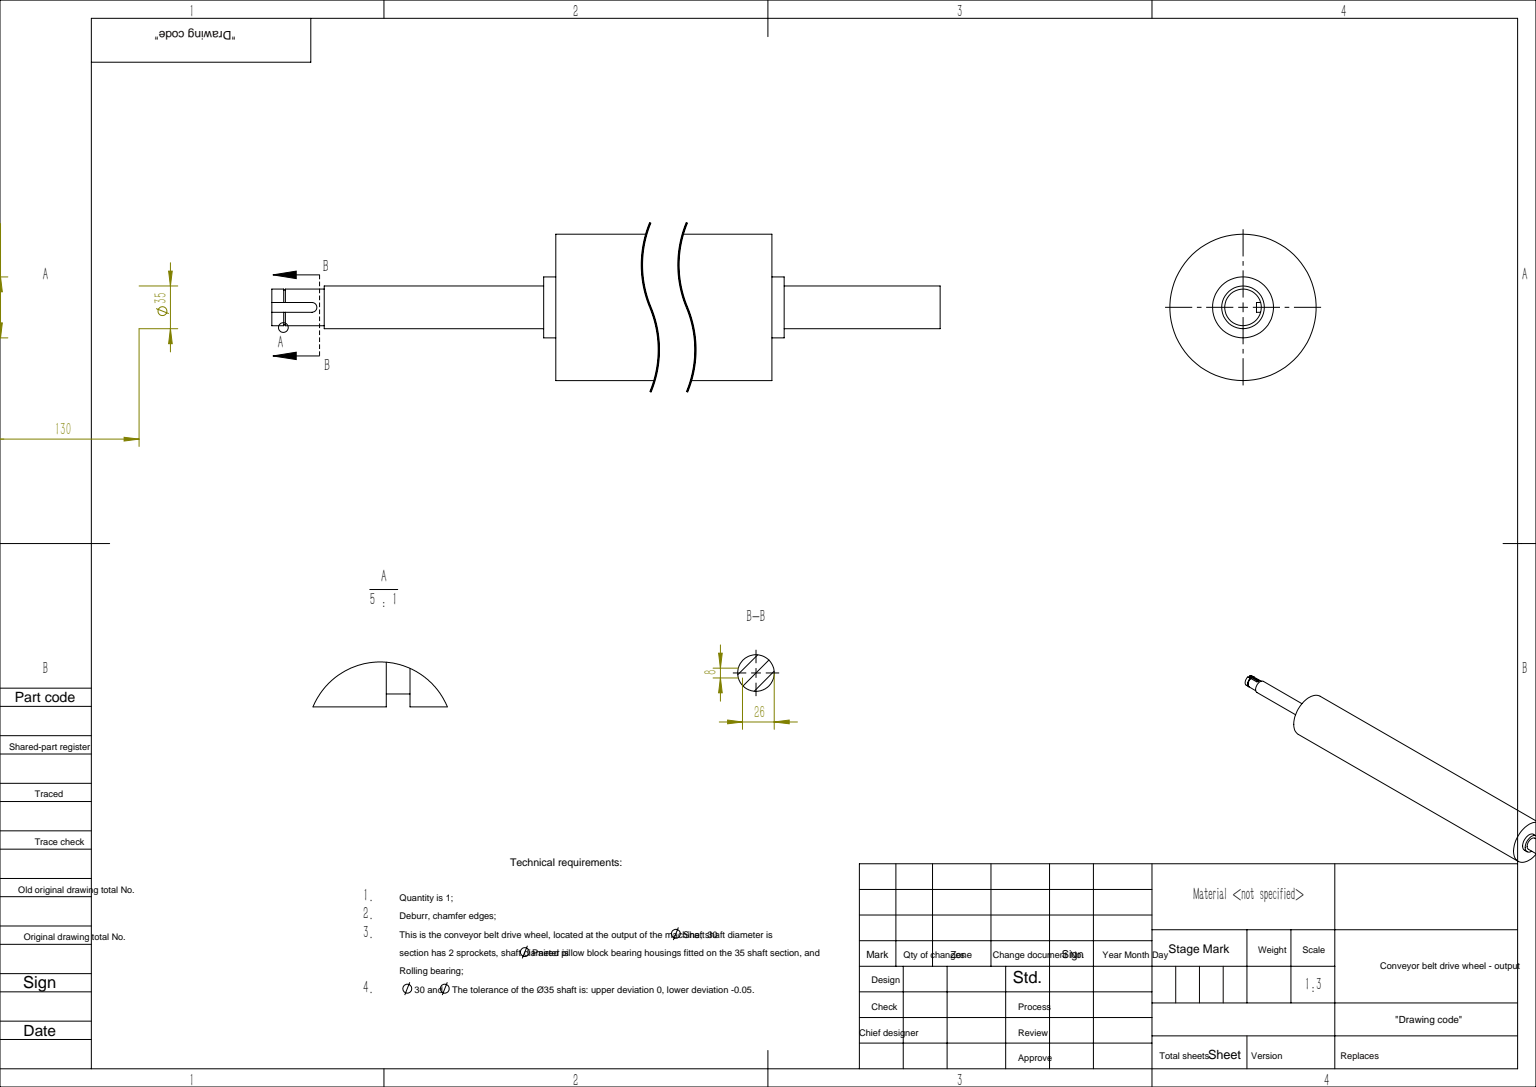
SolidWorks part; units mm, degrees
ref_plane "前视基准面" through (0, 0, 0) normal (0, 0, 1) x (1, 0, 0)
ref_plane "上视基准面" through (0, 0, 0) normal (0, 1, 0) x (1, 0, 0)
ref_plane "右视基准面" through (0, 0, 0) normal (1, 0, 0) x (0, 0, -1)
sketch "草图1" plane through (0, 0, 0) normal (0, 0, 1) x (1, 0, 0)
  line L0 (0, 0) -> (0, 15)
  line L1 (0, 15) -> (43, 15)
  line L2 (43, 15) -> (43, 17.5)
  line L3 (43, 17.5) -> (223, 17.5)
  line L4 (223, 17.5) -> (223, 25)
  line L5 (223, 25) -> (233, 25)
  line L6 (0, 0) -> (1221, 0)
  line L7 (233, 25) -> (233, 60)
  line L8 (233, 60) -> (1083, 60)
  line L9 (1083, 60) -> (1083, 25)
  line L10 (1083, 25) -> (1093, 25)
  line L11 (1093, 25) -> (1093, 17.5)
  line L12 (1093, 17.5) -> (1221, 17.5)
  line L13 (1221, 17.5) -> (1221, 0)
  dimension "D1" = 43
  dimension "D2" = 15
  dimension "D3" = 17.5
  dimension "D4" = 180
  dimension "D5" = 10
  dimension "D6" = 25
  dimension "D7" = 60
  dimension "D8" = 850
  dimension "D9" = 10
  dimension "D10" = 25
  dimension "D11" = 17.5
  dimension "D12" = 128
revolve "旋转1" add sketch "草图1" angle 360 about L6
ref_plane "基准面1" through (0, 15, 0) normal (0, 1, 0) x (1, 0, 0)
sketch "草图2" plane through (0, 15, 0) normal (0, 1, 0) x (1, 0, 0)
  line L0 (0, 0) -> (43, 0) construction
  line L1 (43, 17.5) -> (43, -17.5) construction
  line L2 (33, 4) -> (-10, 4)
  line L3 (-10, 4) -> (-10, -4)
  line L4 (-10, -4) -> (33, -4)
  line L5 (43, 15) -> (43, -15) construction
  line L6 (0, 15) -> (0, -15) construction
  arc A0 (33, -4) -> (33, 4) centre (33, 0) ccw
  dimension "D1" = 4
  dimension "D2" = 10
  dimension "D3" = 10
extrude "切除-拉伸1" cut sketch "草图2" against normal blind 4
ref_plane "基准面2" through (9.8, 0, 0) normal (-1, 0, 0) x (0, 0, 1)
sketch "草图3" plane through (9.8, 0, 0) normal (-1, 0, 0) x (0, 0, 1)
  circle A0 centre (0, 0) radius 15
  arc A2 (-4, 14.4568) -> (4, 14.4568) centre (0, 0) ccw construction
  circle A3 centre (0, 0) radius 14.3
  dimension "D1" = 28.6
extrude "切除-拉伸2" cut sketch "草图3" against normal blind 1.3
